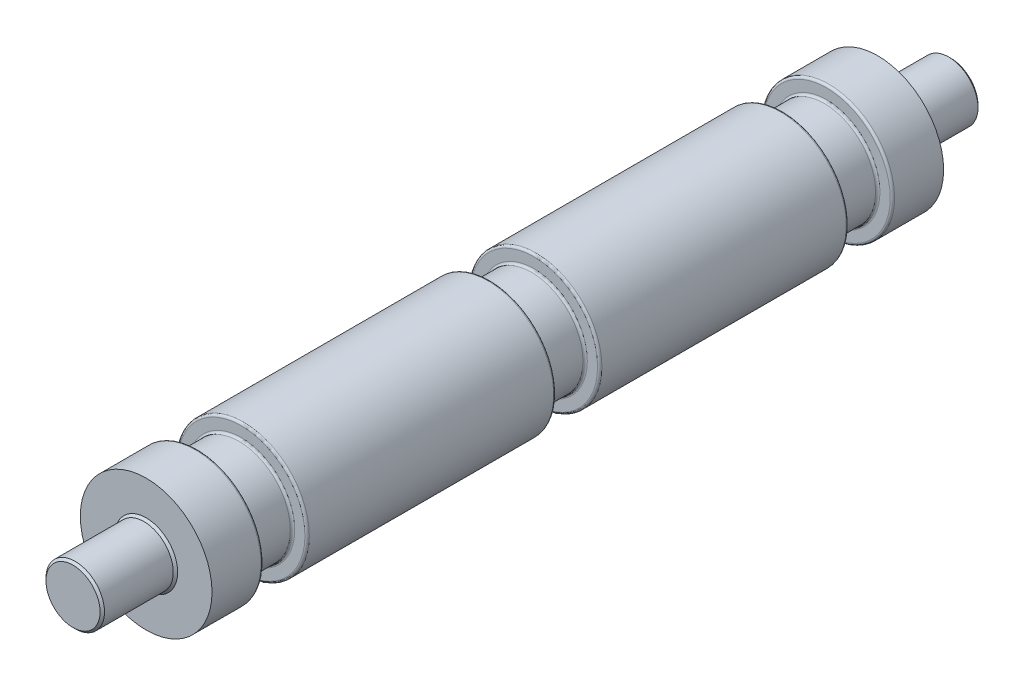
from build123d import *

# Parameters (mm, degrees)
SKETCH1_R                  = 90
BOSS_EXTRUDE1_DEPTH        = 1000
SKETCH2_W                  = 40
SKETCH2_H                  = 60
FILLET1_R                  = 3
LPATTERN1_COUNT            = 2
LPATTERN1_PITCH            = 400
FILLET1_OF_LPATTERN1_R     = 3
LPATTERN1_COL_COUNT        = 2
LPATTERN1_COL_PITCH        = 400
FILLET1_OF_LPATTERN1_COL_R = 3
SKETCH3_R                  = 40
BOSS_EXTRUDE2_DEPTH        = 100
CHAMFER1_SIZE              = 3
BOSS_EXTRUDE3_START        = 100
SKETCH4_R                  = 40
BOSS_EXTRUDE3_DEPTH        = 100
CHAMFER2_SIZE              = 3


with BuildPart() as part:
    # Sketch1 → Boss-Extrude1 (new body)
    with BuildSketch(Plane.XY):
        Circle(SKETCH1_R)
    extrude(amount=BOSS_EXTRUDE1_DEPTH)

    # Sketch2 → Cut-Revolve1 (revolve, cut)
    with BuildSketch(Plane(origin=(0, 0, 0), x_dir=(1, 0, 0), z_dir=(0, 1, 0)), mode=Mode.PRIVATE) as cut_revolve1_sk:
        with Locations((90, -500)):
            Rectangle(SKETCH2_W, SKETCH2_H)
    cut_revolve1 = revolve(cut_revolve1_sk.sketch.rotate(Axis((0, 0, 0), (0, 0, 1)), 180), axis=Axis((0, 0, 0), (0, 0, 1)), mode=Mode.SUBTRACT)

    # Fillet1
    fillet1_edges = [part.edges().sort_by_distance(p)[0] for p in [
        (70, 0, 530),
        (-90, 0, 530),
        (70, 0, 470),
        (-90, 0, 470),
    ]]
    fillet(fillet1_edges, radius=FILLET1_R)

    # LPattern1: Cut-Revolve1 ×2
    with Locations(*[(0, 0, -i * LPATTERN1_PITCH) for i in range(1, LPATTERN1_COUNT)]):
        add(cut_revolve1, mode=Mode.SUBTRACT)

    # Fillet1 of LPattern1
    fillet1_of_lpattern1_edges = [part.edges().sort_by_distance(p)[0] for p in [
        (70, 0, 130),
        (-90, 0, 130),
        (70, 0, 70),
        (-90, 0, 70),
    ]]
    fillet(fillet1_of_lpattern1_edges, radius=FILLET1_OF_LPATTERN1_R)

    # LPattern1 col: Cut-Revolve1 ×2
    with Locations(*[(0, 0, i * LPATTERN1_COL_PITCH) for i in range(1, LPATTERN1_COL_COUNT)]):
        add(cut_revolve1, mode=Mode.SUBTRACT)

    # Fillet1 of LPattern1 col
    fillet1_of_lpattern1_col_edges = [part.edges().sort_by_distance(p)[0] for p in [
        (70, 0, 930),
        (-90, 0, 930),
        (70, 0, 870),
        (-90, 0, 870),
    ]]
    fillet(fillet1_of_lpattern1_col_edges, radius=FILLET1_OF_LPATTERN1_COL_R)

    # Sketch3 → Boss-Extrude2 (add)
    with BuildSketch(Plane.XY.offset(1000)):
        Circle(SKETCH3_R)
    extrude(amount=BOSS_EXTRUDE2_DEPTH)

    # Chamfer1
    chamfer1_edges = [part.edges().sort_by_distance(p)[0] for p in [
        (-40, 0, 1000),
        (-40, 0, 1100),
    ]]
    chamfer(chamfer1_edges, length=CHAMFER1_SIZE)

    # Sketch4 → Boss-Extrude3 (add)
    with BuildSketch(Plane(origin=(0, 0, 0), x_dir=(-1, 0, 0), z_dir=(0, 0, -1)).offset(BOSS_EXTRUDE3_START)):
        with Locations(Location((0, 0, 0), (0, 0, 180))):
            Circle(SKETCH4_R)
    extrude(amount=-BOSS_EXTRUDE3_DEPTH)

    # Chamfer2
    chamfer2_edges = [part.edges().sort_by_distance(p)[0] for p in [
        (-40, 0, 0),
        (-40, 0, -100),
    ]]
    chamfer(chamfer2_edges, length=CHAMFER2_SIZE)


solid = part.part
